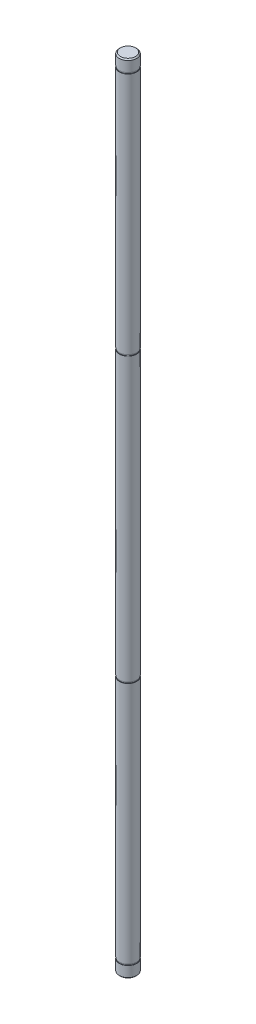
from build123d import *

# Parameters (mm, degrees)
SKETCH1_R           = 7.5
BOSS_EXTRUDE1_DEPTH = 688
SKETCH2_R           = 7.5
SKETCH2_R_2         = 7.15
CUT_EXTRUDE1_DEPTH  = 1.1
CHAMFER1_SIZE       = 1
SKETCH3_R           = 7.5
SKETCH3_R_2         = 7.15
CUT_EXTRUDE2_DEPTH  = 1.1


with BuildPart() as part:
    # Sketch1 → Boss-Extrude1 (new body)
    with BuildSketch(Plane(origin=(0, 0, 0), x_dir=(1, 0, 0), z_dir=(0, 1, 0))):
        with Locations(Location((0, 0, 0), (0, 0, 270))):
            Circle(SKETCH1_R)
    extrude(amount=BOSS_EXTRUDE1_DEPTH)

    # Sketch2 → Cut-Extrude1 (cut)
    with BuildSketch(Plane(origin=(0, 10, 0), x_dir=(-1, 0, 0), z_dir=(0, -1, 0))):
        with Locations(Location((0, 0, 0), (0, 0, 90))):
            Circle(SKETCH2_R)
        with Locations(Location((0, 0, 0), (0, 0, 90))):
            Circle(SKETCH2_R_2, mode=Mode.SUBTRACT)
    cut_extrude1 = extrude(amount=-CUT_EXTRUDE1_DEPTH, mode=Mode.SUBTRACT)

    # Chamfer1
    chamfer1_edges = [part.edges().sort_by_distance(p)[0] for p in [
        (0, 0, -7.5),
        (0, 688, -7.5),
    ]]
    chamfer(chamfer1_edges, length=CHAMFER1_SIZE)

    # Sketch3 → Cut-Extrude2 (cut)
    with BuildSketch(Plane(origin=(0, 221, 0), x_dir=(-1, 0, 0), z_dir=(0, -1, 0))):
        with Locations(Location((0, 0, 0), (0, 0, 90))):
            Circle(SKETCH3_R)
        with Locations(Location((0, 0, 0), (0, 0, 90))):
            Circle(SKETCH3_R_2, mode=Mode.SUBTRACT)
    cut_extrude2 = extrude(amount=-CUT_EXTRUDE2_DEPTH, mode=Mode.SUBTRACT)

    # Mirror1: Cut-Extrude1, Cut-Extrude2 across plane
    add(cut_extrude1.mirror(Plane(origin=(0, 344, 0), x_dir=(0, 0, 1), z_dir=(0, -1, 0))), mode=Mode.SUBTRACT)
    add(cut_extrude2.mirror(Plane(origin=(0, 344, 0), x_dir=(0, 0, 1), z_dir=(0, -1, 0))), mode=Mode.SUBTRACT)


solid = part.part
